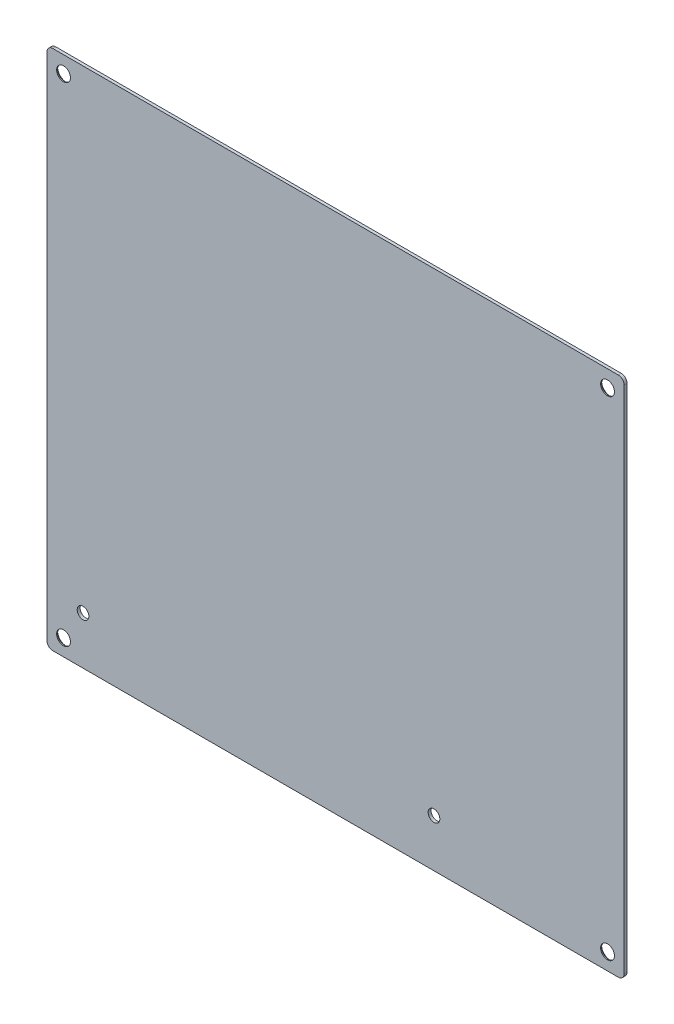
from build123d import *

# Parameters (mm, degrees)
SKETCH_1_W          = 296
SKETCH_1_H          = 267.5
EXTRUDE_1_DEPTH     = 1.5
FILLET_1_R          = 3
SKETCH_6_R          = 3
CUT_EXTRUDE_1_DEPTH = 1.5
SKETCH_7_R          = 3.55
CUT_EXTRUDE_2_DEPTH = 1.5
CHAMFER_1_SIZE      = 1


with BuildPart() as part:
    # 草图1 → 凸台-拉伸1 (new body)
    with BuildSketch(Plane.XY):
        with Locations((-237.5, 200.75)):
            Rectangle(SKETCH_1_W, SKETCH_1_H)
    extrude(amount=-EXTRUDE_1_DEPTH)

    # 圆角1
    fillet_1_edges = [part.edges().sort_by_distance(p)[0] for p in [
        (-385.5, 67, -0.75),
        (-385.5, 334.5, -0.75),
        (-89.5, 334.5, -0.75),
        (-89.5, 67, -0.75),
    ]]
    fillet(fillet_1_edges, radius=FILLET_1_R)

    # 草图6 → 切除-拉伸1 (cut)
    with BuildSketch(Plane.XY):
        with Locations((-367, 91.5)):
            Circle(SKETCH_6_R)
        with Locations((-187, 91.5)):
            Circle(SKETCH_6_R)
    extrude(amount=-CUT_EXTRUDE_1_DEPTH, mode=Mode.SUBTRACT)

    # 草图7 → 切除-拉伸2 (cut)
    with BuildSketch(Plane(origin=(0, 0, -1.5), x_dir=(-1, 0, 0), z_dir=(0, 0, -1))):
        with Locations((98, 326)):
            Circle(SKETCH_7_R)
        with Locations((377, 326)):
            Circle(SKETCH_7_R)
        with Locations((377, 75.5)):
            Circle(SKETCH_7_R)
        with Locations((98, 75.5)):
            Circle(SKETCH_7_R)
    extrude(amount=-CUT_EXTRUDE_2_DEPTH, mode=Mode.SUBTRACT)

    # 倒角1
    chamfer_1_edges = [part.edges().sort_by_distance(p)[0] for p in [
        (-94.45, 326, -1.5),
        (-373.45, 326, -1.5),
        (-373.45, 75.5, -1.5),
        (-94.45, 75.5, -1.5),
    ]]
    chamfer(chamfer_1_edges, length=CHAMFER_1_SIZE)


solid = part.part
